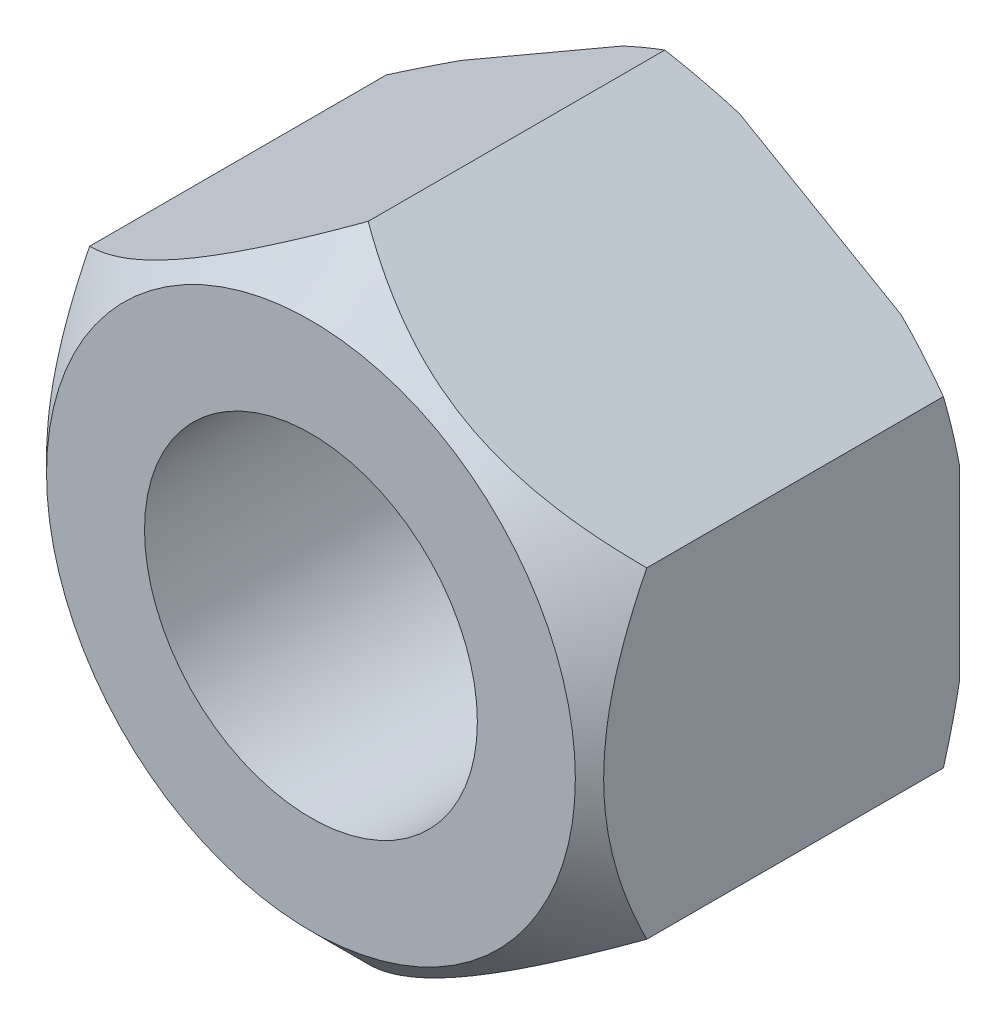
SolidWorks part; units mm, degrees
ref_plane "基准面1" through (0, 0, 0) normal (0, 0, 1) x (1, 0, 0)
ref_plane "基准面2" through (0, 0, 0) normal (0, 1, 0) x (1, 0, 0)
ref_plane "基准面3" through (0, 0, 0) normal (1, 0, 0) x (0, 0, -1)
sketch "尺寸草图" plane through (0, 0, 0) normal (0, 0, 1) x (1, 0, 0)
  line L0 (0, 0) -> (44.4, 0)
  line L1 (0, 0) -> (19.5, 0)
  line L2 (19.5, 0) -> (44.4, 0)
  line L3 (-17.1429, 0) -> (0, 0)
  point P3 (18, 0)
  point P4 (2.5, 0)
  point P5 (29.56, 0)
  point P7 (12.08, 0)
  point P8 (27, 0)
  point P15 (36.5, 0)
  dimension "D1" = 17.1429
  dimension "D" = 18
  dimension "P" = 2.5
  dimension "e(min)" = 29.56
  dimension "mw(min)" = 12.08
  dimension "s(max)" = 27
  dimension "da(max)" = 19.5
  dimension "dw(min)" = 24.9
  dimension "h(max)" = 17
sketch "草图1" plane through (0, 0, 0) normal (0, 0, 1) x (1, 0, 0)
  line L0 (-12.7999, 0) -> (12.7999, 0) construction
  line L1 (0, 14.78) -> (0, -14.78) construction
  line L3 (0, 14.78) -> (-12.7999, 7.39)
  line L4 (-12.7999, 7.39) -> (-12.7999, -7.39)
  line L5 (-12.7999, -7.39) -> (0, -14.78)
  line L6 (0, -14.78) -> (12.7999, -7.39)
  line L7 (12.7999, -7.39) -> (12.7999, 7.39)
  line L8 (12.7999, 7.39) -> (0, 14.78)
  circle A0 centre (0, 0) radius 12.7999 construction
  circle A1 centre (0, 0) radius 7.6469
  dimension "D" = 15.2937
  dimension "e" = 29.56
extrude "基体-拉伸" add sketch "草图1" along normal blind 17
cosmetic thread "装饰螺纹线1" parameters "D2"=18
sketch "草图2" plane through (0, 0, 0) normal (0, 0, -1) x (-1, 0, 0)
  circle A0 centre (0, 0) radius 13.5
  circle A1 centre (0, 0) radius 7.6469 construction
  dimension "s" = 27
extrude "切除-拉伸1" cut sketch "草图2" against normal through all draft 60 flip side to cut
chamfer "倒角1" distance 0.2946 angle 45 1 edges at (7.6469, 0, 0)
sketch "草图9" plane through (0, 0, 17) normal (0, 0, 1) x (1, 0, 0)
  circle A0 centre (0, 0) radius 12.15
  dimension "s*0.9" = 24.3
extrude "切除-拉伸7" cut sketch "草图9" against normal through all draft 45 flip side to cut
